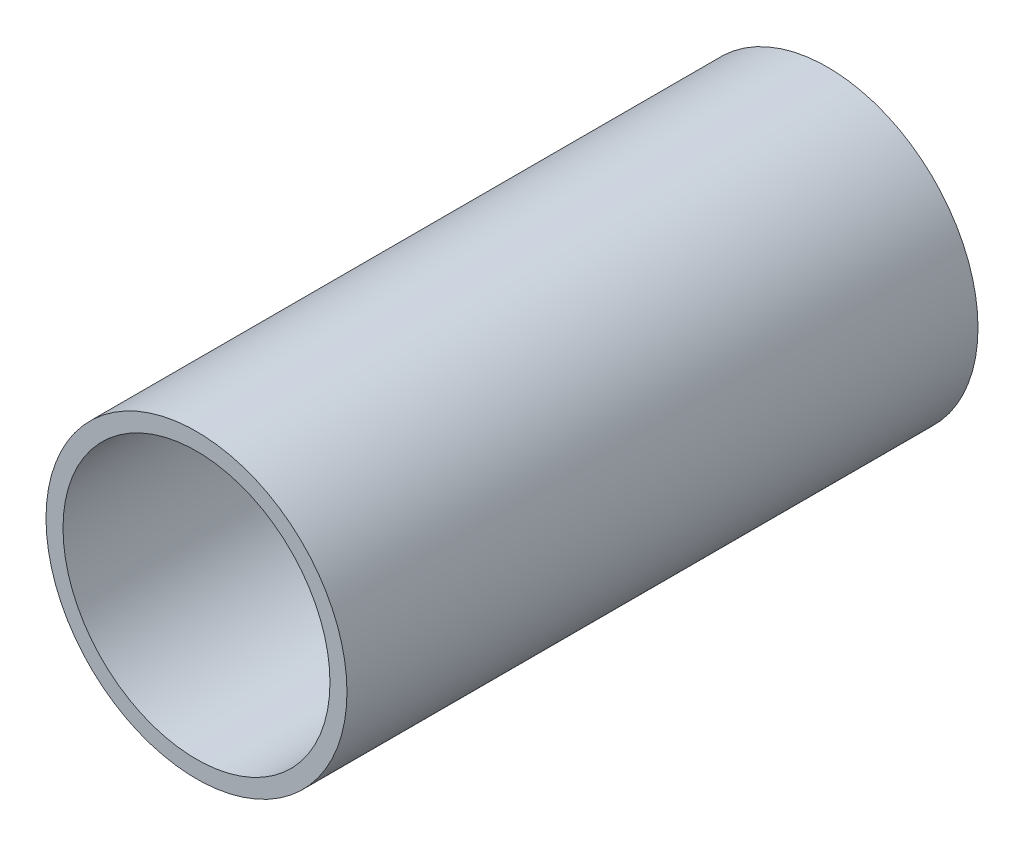
SolidWorks part; units mm, degrees
ref_plane "前视基准面" through (0, 0, 0) normal (0, 0, 1) x (1, 0, 0)
ref_plane "上视基准面" through (0, 0, 0) normal (0, 1, 0) x (1, 0, 0)
ref_plane "右视基准面" through (0, 0, 0) normal (1, 0, 0) x (0, 0, -1)
sketch "草图1" plane through (0, 0, 0) normal (0, 0, 1) x (1, 0, 0)
  circle A0 centre (0, 0) radius 27.5
  circle A1 centre (0, 0) radius 31
  dimension "D1" = 55
  dimension "D2" = 62
extrude "凸台-拉伸1" add sketch "草图1" along normal blind 130
